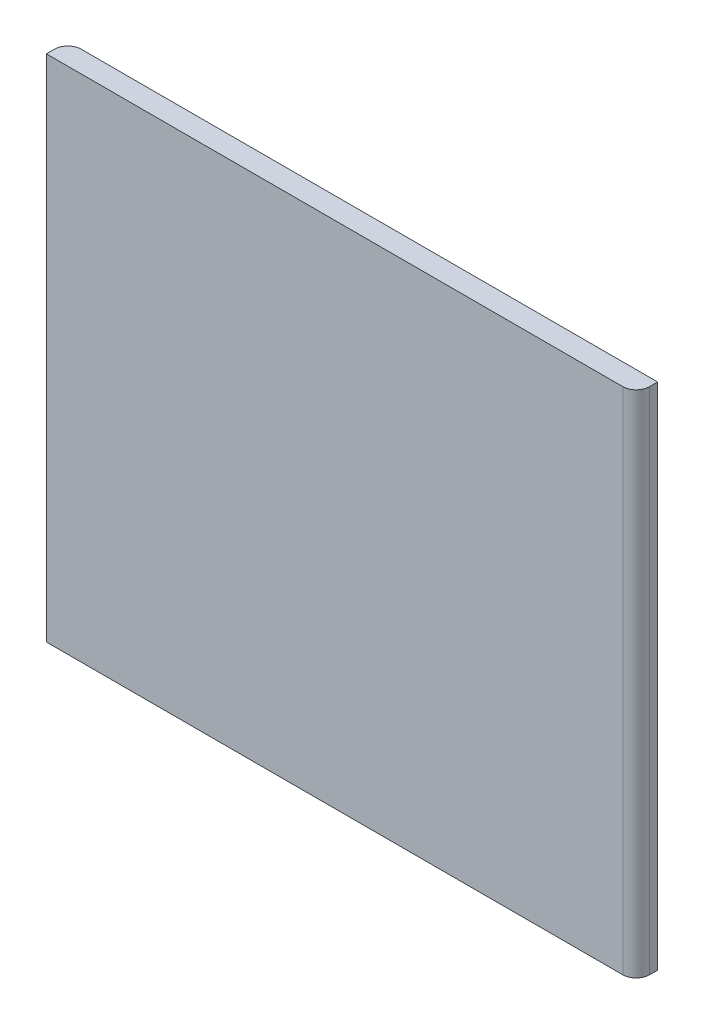
from build123d import *

# Parameters (mm, degrees)
SKETCH1_W           = 220
SKETCH1_H           = 190
BOSS_EXTRUDE1_DEPTH = 8
FILLET1_R           = 5


with BuildPart() as part:
    # Sketch1 → Boss-Extrude1 (new body)
    with BuildSketch(Plane.XY):
        Rectangle(SKETCH1_W, SKETCH1_H)
    extrude(amount=BOSS_EXTRUDE1_DEPTH)

    # Fillet1
    fillet1_edges = [part.edges().sort_by_distance(p)[0] for p in [
        (110, 0, 8),
        (-110, 0, 0),
    ]]
    fillet(fillet1_edges, radius=FILLET1_R)


solid = part.part
